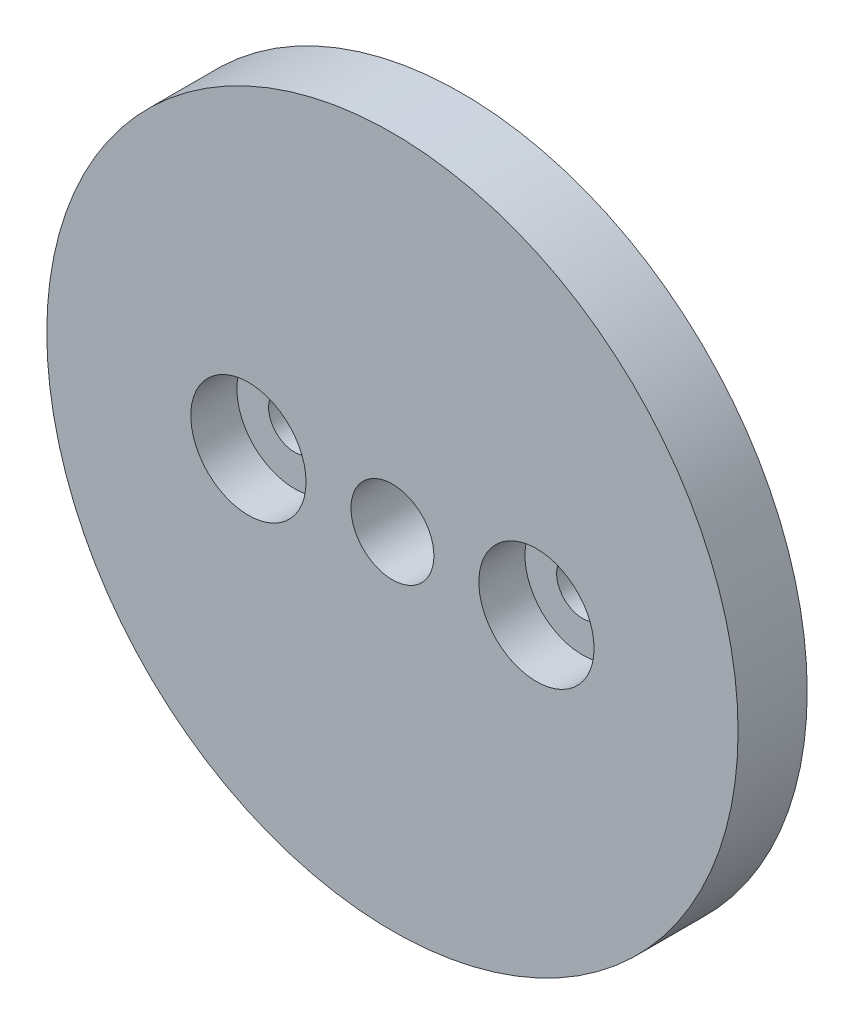
from build123d import *

# Parameters (mm, degrees)
SKETCH1_R                               = 30
BOSS_EXTRUDE1_DEPTH                     = 6
CBORE_FOR_M4_HEX_HEAD_BOLT1_D           = 4.5
CBORE_FOR_M4_HEX_HEAD_BOLT1_CBORE_D     = 10
CBORE_FOR_M4_HEX_HEAD_BOLT1_CBORE_DEPTH = 4
SKETCH4_R                               = 3.6
CUT_EXTRUDE1_DEPTH                      = 10


with BuildPart() as part:
    # Sketch1 → Boss-Extrude1 (new body)
    with BuildSketch(Plane.XY):
        Circle(SKETCH1_R)
    extrude(amount=BOSS_EXTRUDE1_DEPTH)

    # CBORE for M4 Hex Head Bolt1 (through all)
    with Locations(Plane.XY.offset(6)):
        with Locations((-12.5, 0), (12.5, 0)):
            CounterBoreHole(CBORE_FOR_M4_HEX_HEAD_BOLT1_D / 2, CBORE_FOR_M4_HEX_HEAD_BOLT1_CBORE_D / 2, CBORE_FOR_M4_HEX_HEAD_BOLT1_CBORE_DEPTH)

    # Sketch4 → Cut-Extrude1 (cut)
    with BuildSketch(Plane.XY.offset(6)):
        Circle(SKETCH4_R)
    extrude(amount=-CUT_EXTRUDE1_DEPTH, mode=Mode.SUBTRACT)


solid = part.part
